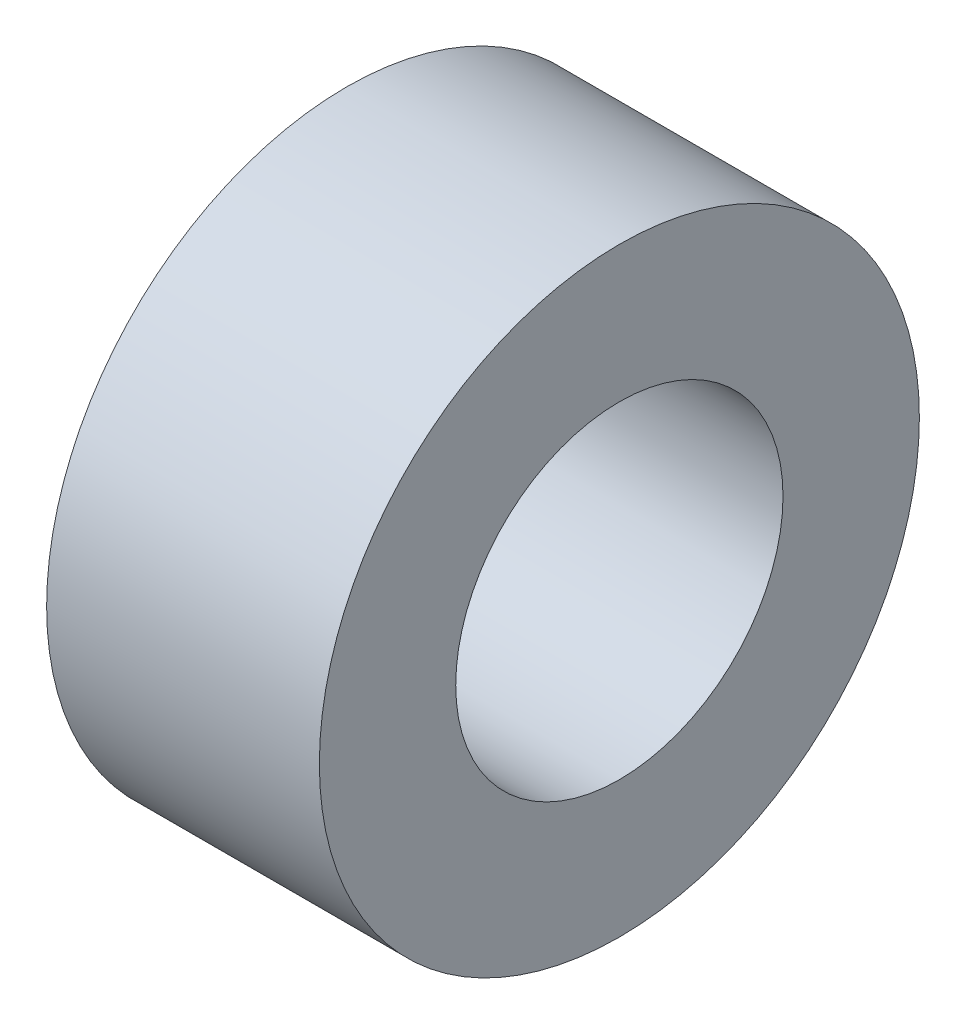
from build123d import *

# Parameters (mm, degrees)
SKETCH1_R           = 5.5
SKETCH1_R_2         = 3
BOSS_EXTRUDE1_DEPTH = 5


with BuildPart() as part:
    # Sketch1 → Boss-Extrude1 (new body)
    with BuildSketch(Plane(origin=(0, 0, 0), x_dir=(0, 0, -1), z_dir=(1, 0, 0))):
        Circle(SKETCH1_R)
        Circle(SKETCH1_R_2, mode=Mode.SUBTRACT)
    extrude(amount=BOSS_EXTRUDE1_DEPTH)


solid = part.part
